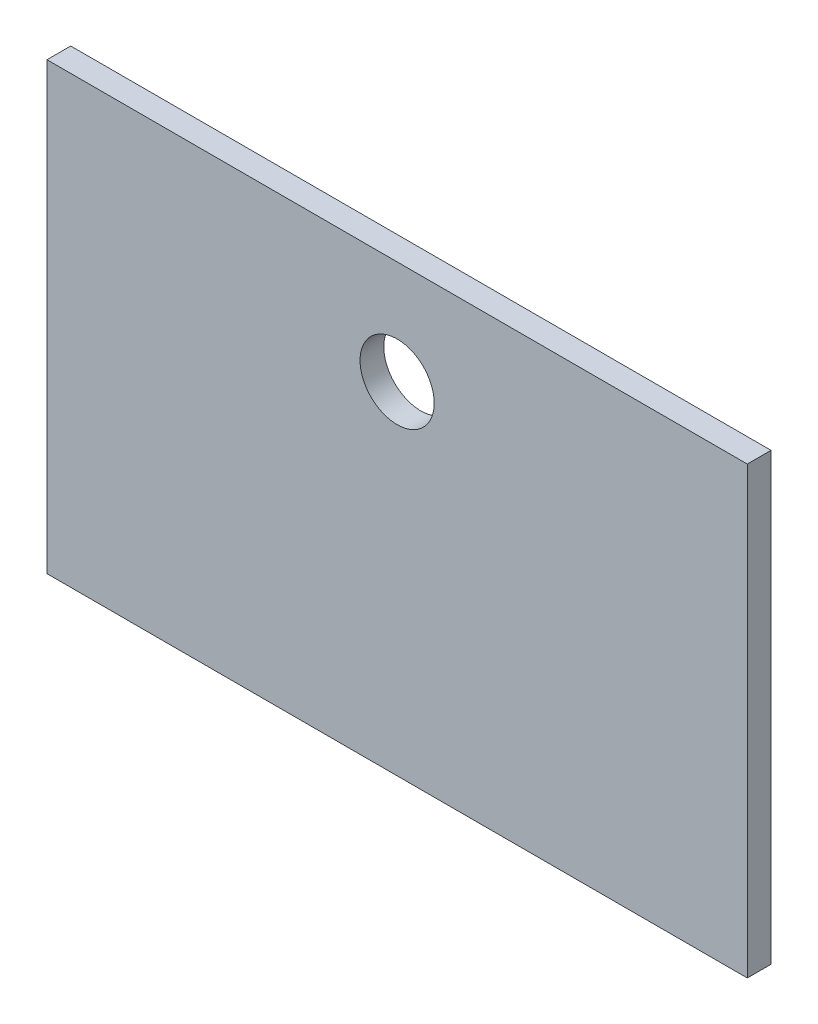
SolidWorks part; units mm, degrees
material "Q235B"
ref_plane "Front Plane" through (0, 0, 0) normal (0, 0, 1) x (1, 0, 0)
ref_plane "Top Plane" through (0, 0, 0) normal (0, 1, 0) x (1, 0, 0)
ref_plane "Right Plane" through (0, 0, 0) normal (1, 0, 0) x (0, 0, -1)
sketch "Sketch1" plane through (0, 0, 0) normal (0, 0, 1) x (1, 0, 0)
  line L1 (118, -75) -> (-118, -75)
  line L2 (118, -75) -> (118, 75)
  line L3 (118, 75) -> (-118, 75)
  line L4 (-118, -75) -> (-118, 75)
  line L5 (118, -75) -> (-118, 75) construction
  line L6 (118, 75) -> (-118, -75) construction
  point P0 (0, 0)
  dimension "D1" = 150
  dimension "D2" = 236
extrude "Boss-Extrude1" add sketch "Sketch1" along normal mid plane 8
hole_wizard "Ø25.0 (25) Diameter Hole1" positions "Sketch2" profile "Sketch3" hole size "Ø25.0" standard "GB" end condition up to next
sketch "Sketch2" plane through (0, 0, 4) normal (0, 0, 1) x (1, 0, 0)
  line L0 (0, 29.1317) -> (0, 40) construction
  line L1 (0, 40) -> (-59.2649, 40) construction
  line L2 (-118, -75) -> (118, -75) construction
  point P4 (0, 40)
  dimension "D1" = 115
sketch "Sketch3" plane through (0, 40, 4) normal (1, 0, 0) x (0, -1, 0)
  line L0 (0, 0) -> (0, 8)
  line L1 (0, 8) -> (12.5, 8)
  line L2 (12.5, 8) -> (12.5, 0)
  line L5 (12.5, 0) -> (0, 0)
  line L11 (0, -6.35) -> (0, 107.95) construction
  dimension "通孔孔直径" = 25
  dimension "通孔孔深度" = 8
